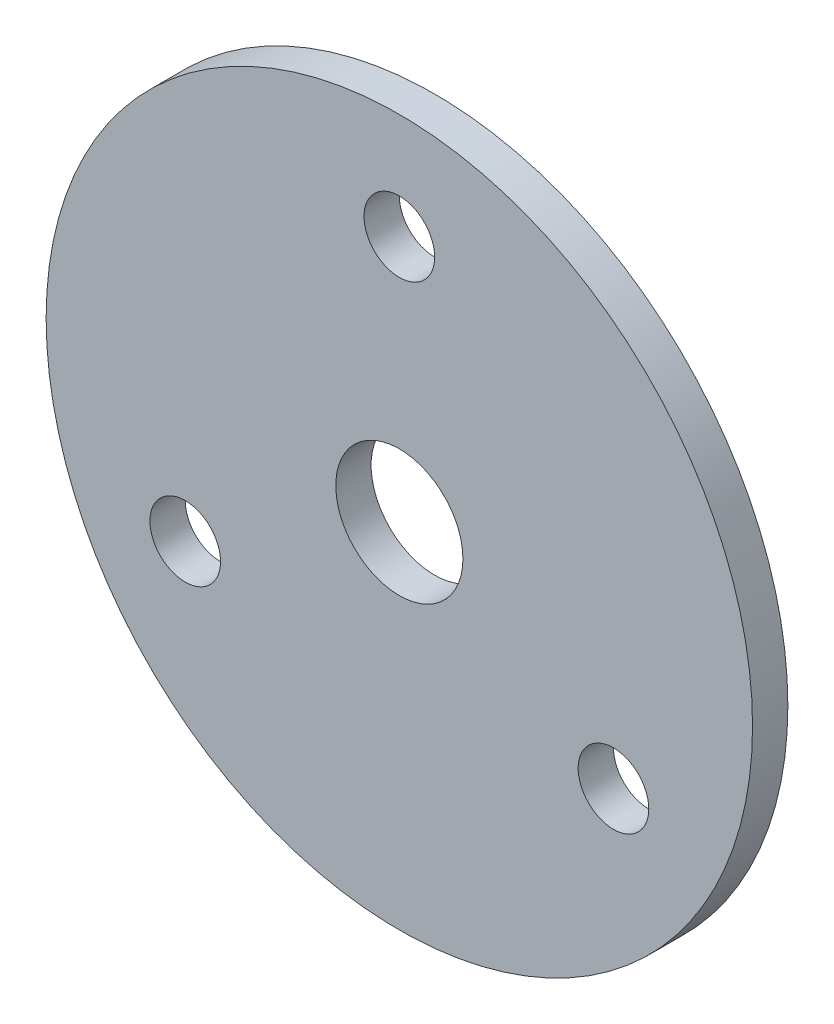
SolidWorks part; units mm, degrees
ref_plane "Front Plane" through (0, 0, 0) normal (0, 0, 1) x (1, 0, 0)
ref_plane "Top Plane" through (0, 0, 0) normal (0, 1, 0) x (1, 0, 0)
ref_plane "Right Plane" through (0, 0, 0) normal (1, 0, 0) x (0, 0, -1)
other "Configuration Table"
sketch "Sketch1" plane through (0, 0, 0) normal (0, 0, 1) x (1, 0, 0)
  circle A0 centre (0, 0) radius 50
  dimension "D1" = 100
extrude "Boss-Extrude1" add sketch "Sketch1" along normal blind 5
sketch "Sketch2" plane through (0, 0, 5) normal (0, 0, 1) x (1, 0, 0)
  circle A1 centre (0, 35) radius 5
  dimension "D1" = 35
  dimension "D2" = 10
extrude "Cut-Extrude1" cut sketch "Sketch2" against normal blind 5
pattern_circular "CirPattern1" count 3 over 360 about axis through (0, 0, 0) along (0, 0, 1) of "Cut-Extrude1"
sketch "Sketch3" plane through (0, 0, 5) normal (0, 0, 1) x (1, 0, 0)
  circle A0 centre (0, 0) radius 9
  dimension "D1" = 18
extrude "Cut-Extrude2" cut sketch "Sketch3" against normal blind 5
